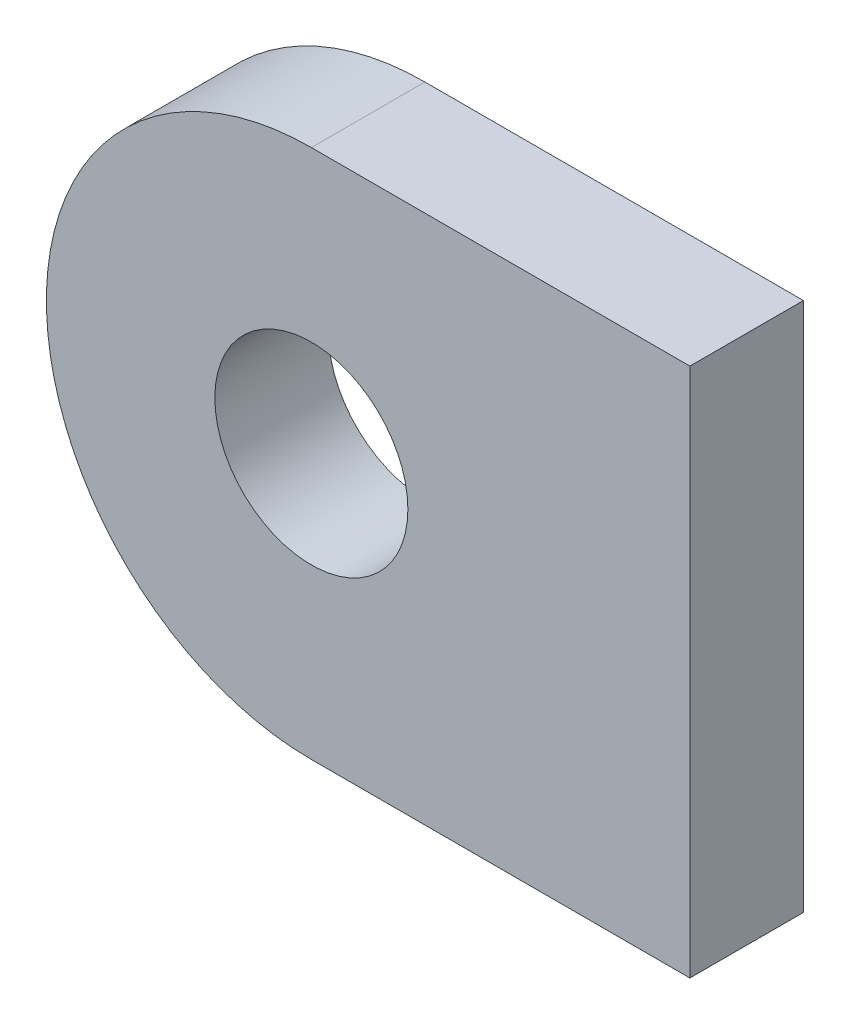
SolidWorks part; units mm, degrees
ref_plane "前视基准面" through (0, 0, 0) normal (0, 0, 1) x (1, 0, 0)
ref_plane "上视基准面" through (0, 0, 0) normal (0, 1, 0) x (1, 0, 0)
ref_plane "右视基准面" through (0, 0, 0) normal (1, 0, 0) x (0, 0, -1)
other "Configuration Table"
sketch "草图1" plane through (0, 0, 0) normal (0, 0, 1) x (1, 0, 0)
  line L0 (0, 14) -> (20, 14)
  line L1 (20, 14) -> (20, -14)
  line L2 (20, -14) -> (0, -14)
  arc A0 (0, -14) -> (0, 14) centre (0, 0) cw
  circle A1 centre (0, 0) radius 5.1
  point P0 (0, 0)
  dimension "D1" = 10.2
  dimension "D2" = 14
  dimension "D3" = 20
extrude "凸台-拉伸1" add sketch "草图1" against normal mid plane 6
